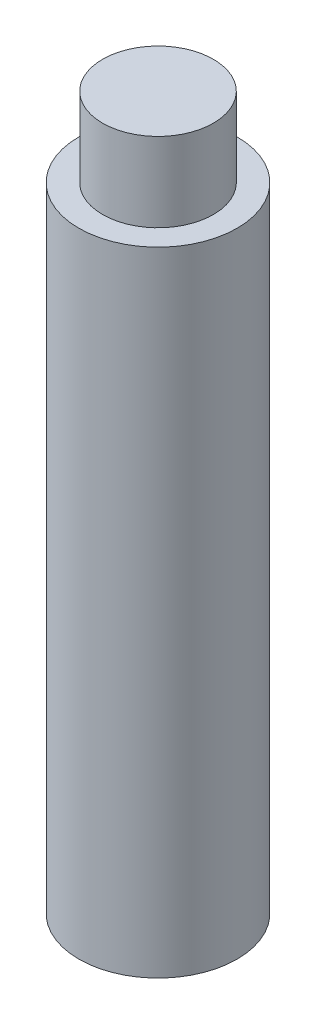
SolidWorks part; units mm, degrees
ref_plane "Front Plane" through (0, 0, 0) normal (0, 0, 1) x (1, 0, 0)
ref_plane "Top Plane" through (0, 0, 0) normal (0, 1, 0) x (1, 0, 0)
ref_plane "Right Plane" through (0, 0, 0) normal (1, 0, 0) x (0, 0, -1)
other "Configuration Table"
sketch "Sketch1" plane through (0, 0, 0) normal (0, 1, 0) x (1, 0, 0)
  circle A0 centre (0, 0) radius 10
  dimension "D1" = 20
extrude "Boss-Extrude1" add sketch "Sketch1" along normal blind 5
sketch "Sketch2" plane through (0, 5, 0) normal (0, 1, 0) x (1, 0, 0)
  circle A0 centre (0, 0) radius 10
  dimension "D1" = 20
extrude "Boss-Extrude2" add sketch "Sketch2" along normal blind 75 contours A0
sketch "Sketch3" plane through (0, 80, 0) normal (0, 1, 0) x (1, 0, 0)
  circle A0 centre (0, 0) radius 7
  dimension "D1" = 14
extrude "Boss-Extrude3" add sketch "Sketch3" along normal blind 10
ref_plane "Plane1" through (10, 0, 0) normal (1, 0, 0) x (0, 0, -1)
sketch "Sketch5" plane through (10, 0, 0) normal (1, 0, 0) x (0, 0, -1)
  line L0 (10, 0) -> (10, 80) construction
  line L1 (-10, 0) -> (10, 0)
  line L2 (-10, 0) -> (-10, 18)
  line L3 (-10, 18) -> (10, 18)
  line L4 (10, 0) -> (10, 18)
  dimension "D1" = 18
extrude "Cut-Extrude1" [suppressed] cut sketch "Sketch5" against normal blind 2.5
ref_plane "Plane2" through (0, 0, 0) normal (1, 0, 0) x (0, 0, -1)
mirror "Mirror1" [suppressed] about plane through (0, 0, 0) normal (1, 0, 0)
sketch "Sketch6" [suppressed] plane through (7.5, 0, 0) normal (1, 0, 0) x (0, 0, -1)
  line L0 (6.6144, 0) -> (-6.6144, 0) construction
  circle A0 centre (0, 5) radius 3.5
  dimension "D1" = 7
  dimension "D2" = 5
extrude "Cut-Extrude2" [suppressed] cut sketch "Sketch6" against normal through all
